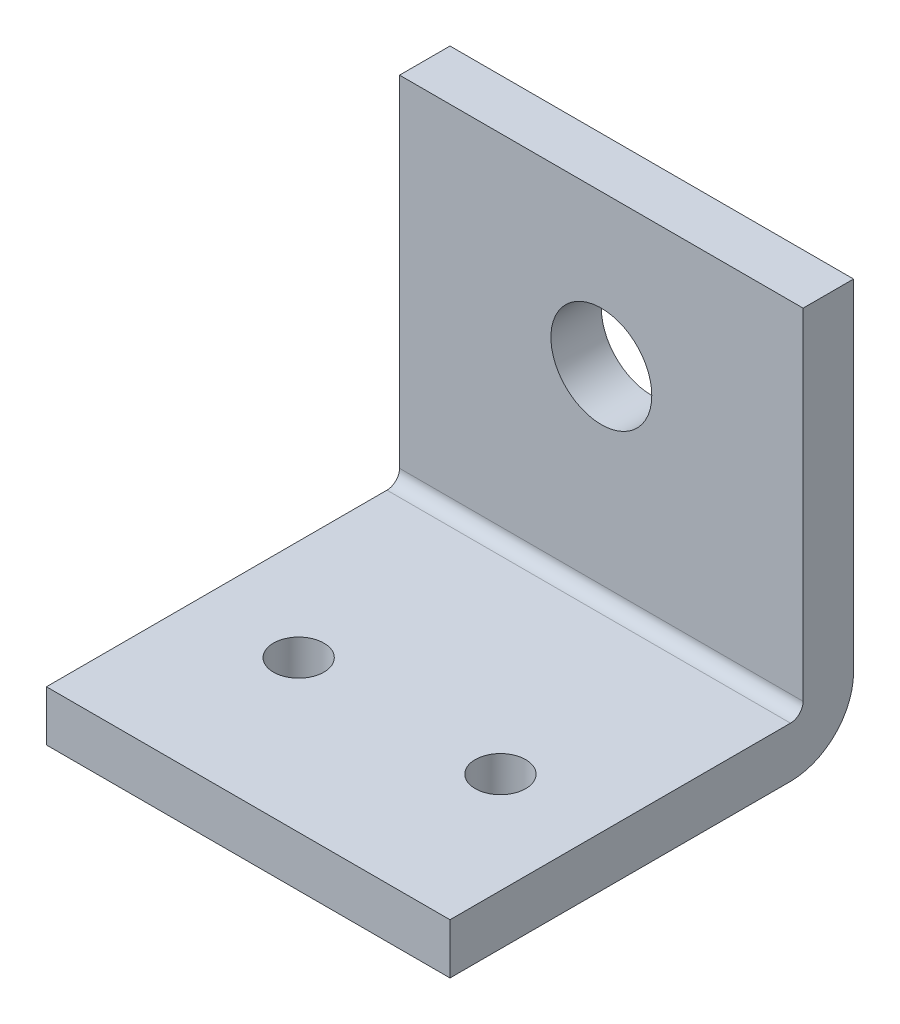
from build123d import *

# Parameters (mm, degrees)
BOSS_EXTRUDE1_DEPTH = 40
SKETCH2_R           = 5
CUT_EXTRUDE1_DEPTH  = 40
SKETCH3_R           = 2.5
CUT_EXTRUDE2_DEPTH  = 40


with BuildPart() as part:
    # Sketch1 → Boss-Extrude1 (new body)
    with BuildSketch(Plane(origin=(0, 0, 0), x_dir=(0, 0, -1), z_dir=(1, 0, 0))):
        with BuildLine():
            Line((11.805555556, 25.625), (11.805555556, -8.125))
            ThreePointArc((11.805555556, -8.125), (11.439439032, -9.008883476), (10.555555556, -9.375))
            Line((10.555555556, -9.375), (-23.194444444, -9.375))
            Line((-23.194444444, -9.375), (-23.194444444, -14.375))
            Line((-23.194444444, -14.375), (10.555555556, -14.375))
            ThreePointArc((10.555555556, -14.375), (14.974972938, -12.544417382), (16.805555556, -8.125))
            Line((16.805555556, -8.125), (16.805555556, 25.625))
            Line((16.805555556, 25.625), (11.805555556, 25.625))
        make_face()
    extrude(amount=-BOSS_EXTRUDE1_DEPTH)

    # Sketch2 → Cut-Extrude1 (cut)
    with BuildSketch(Plane.XY.offset(-11.805555556)):
        with Locations((-20, 10.625)):
            Circle(SKETCH2_R)
    extrude(amount=-CUT_EXTRUDE1_DEPTH, mode=Mode.SUBTRACT)

    # Sketch3 → Cut-Extrude2 (cut)
    with BuildSketch(Plane(origin=(0, -9.375, 0), x_dir=(1, 0, 0), z_dir=(0, 1, 0))):
        with Locations(Location((-30, -8.194444444, 0), (0, 0, 270))):
            Circle(SKETCH3_R)
        with Locations(Location((-10, -8.194444444, 0), (0, 0, 270))):
            Circle(SKETCH3_R)
    extrude(amount=-CUT_EXTRUDE2_DEPTH, mode=Mode.SUBTRACT)


solid = part.part
